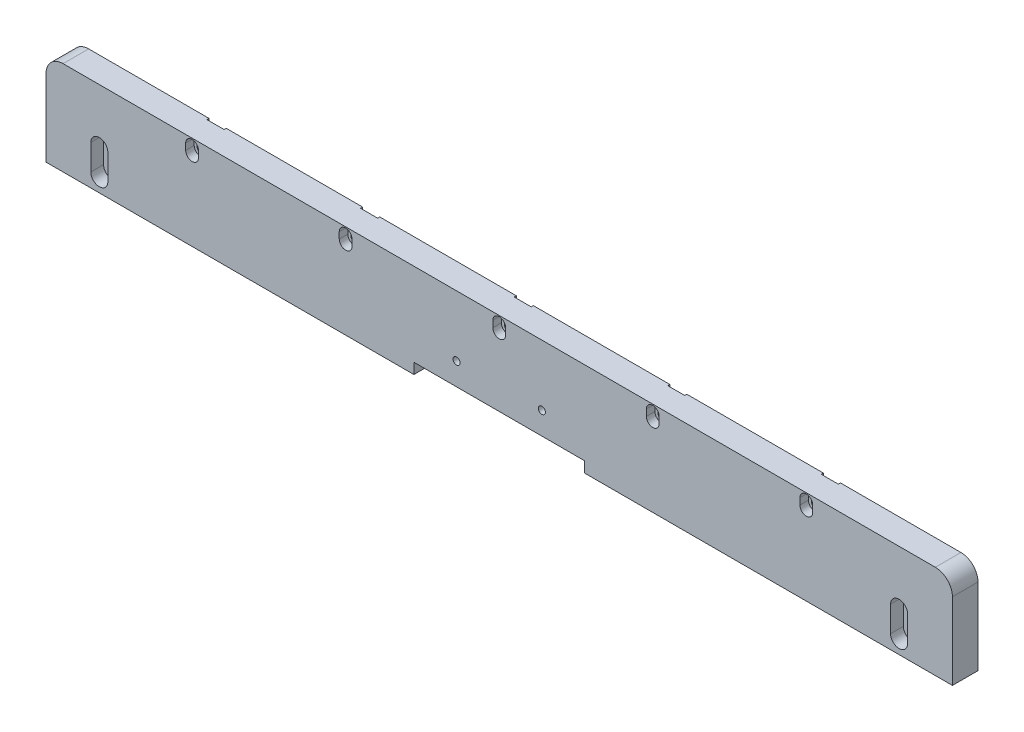
SolidWorks part; units mm, degrees
ref_plane "前视基准面" through (0, 0, 0) normal (0, 0, 1) x (1, 0, 0)
ref_plane "上视基准面" through (0, 0, 0) normal (0, 1, 0) x (1, 0, 0)
ref_plane "右视基准面" through (0, 0, 0) normal (1, 0, 0) x (0, 0, -1)
sketch "草图1" plane through (0, 0, 0) normal (0, 0, 1) x (1, 0, 0)
  line L1 (-212.5, 22) -> (212.5, 22)
  line L2 (-212.5, 22) -> (-212.5, -22)
  line L3 (-212.5, -22) -> (212.5, -22)
  line L4 (212.5, 22) -> (212.5, -22)
  line L5 (-212.5, 22) -> (212.5, -22) construction
  line L6 (-212.5, -22) -> (212.5, 22) construction
  point P0 (0, 0)
  dimension "D1" = 425
  dimension "D2" = 44
extrude "凸台-拉伸1" add sketch "草图1" along normal blind 12
fillet "圆角1" radius 8 2 edges at (212.5, 22, 6) (-212.5, 22, 6)
sketch "草图2" plane through (0, 0, 12) normal (0, 0, 1) x (1, 0, 0)
  line L0 (-187.5, -3.5) -> (-187.5, -15.5) construction
  line L1 (-183.5, -3.5) -> (-183.5, -15.5)
  line L2 (-191.5, -3.5) -> (-191.5, -15.5)
  line L3 (-212.5, 14) -> (-212.5, -22) construction
  line L4 (-212.5, -22) -> (212.5, -22) construction
  line L6 (0, 45.6197) -> (0, -20.1141) construction
  line L7 (187.5, -3.5) -> (187.5, -15.5) construction
  line L8 (183.5, -3.5) -> (183.5, -15.5)
  line L9 (191.5, -3.5) -> (191.5, -15.5)
  arc A0 (-183.5, -3.5) -> (-191.5, -3.5) centre (-187.5, -3.5) ccw
  arc A1 (-191.5, -15.5) -> (-183.5, -15.5) centre (-187.5, -15.5) ccw
  arc A2 (183.5, -3.5) -> (191.5, -3.5) centre (187.5, -3.5) cw
  arc A3 (191.5, -15.5) -> (183.5, -15.5) centre (187.5, -15.5) cw
  point P2 (-187.5, -9.5)
  point P16 (187.5, -9.5)
  dimension "D4" = 4
  dimension "D1" = 25
  dimension "D2" = 6.5
  dimension "D3" = 12
extrude "切除-拉伸1" cut sketch "草图2" against normal blind 6
sketch "草图3" plane through (0, 0, 6) normal (0, 0, 1) x (1, 0, 0)
  line L0 (-187.5, -3.5) -> (-187.5, -15.5) construction
  line L1 (-185.5, -3.5) -> (-185.5, -15.5)
  line L2 (-189.5, -3.5) -> (-189.5, -15.5)
  line L3 (187.5, -3.5) -> (187.5, -15.5) construction
  line L4 (189.5, -3.5) -> (189.5, -15.5)
  line L5 (185.5, -3.5) -> (185.5, -15.5)
  arc A0 (-185.5, -3.5) -> (-189.5, -3.5) centre (-187.5, -3.5) ccw
  arc A1 (-189.5, -15.5) -> (-185.5, -15.5) centre (-187.5, -15.5) ccw
  arc A2 (189.5, -3.5) -> (185.5, -3.5) centre (187.5, -3.5) ccw
  arc A3 (185.5, -15.5) -> (189.5, -15.5) centre (187.5, -15.5) ccw
  point P4 (-187.5, -9.5)
  point P13 (187.5, -9.5)
  dimension "D1" = 2
  dimension "D2" = 2
extrude "切除-拉伸2" cut sketch "草图3" against normal through all
sketch "草图8" plane through (0, 0, 12) normal (0, 0, 1) x (1, 0, 0)
  line L0 (-212.5, -22) -> (212.5, -22) construction
  line L1 (40, -17) -> (-40, -17)
  line L2 (40, -17) -> (40, -52.5185)
  line L3 (40, -52.5185) -> (-40, -52.5185)
  line L4 (-40, -17) -> (-40, -52.5185)
  line L5 (40, -17) -> (-40, -52.5185) construction
  line L6 (40, -52.5185) -> (-40, -17) construction
  line L7 (0, 36.33) -> (0, -6.1683) construction
  point P0 (0, -34.7592)
  point P10 (0, -17)
  dimension "D1" = 5
  dimension "D2" = 80
extrude "切除-拉伸3" cut sketch "草图8" against normal through all
sketch "草图10" plane through (0, 0, 0) normal (0, 0, -1) x (-1, 0, 0)
  line L0 (-204.5, 22) -> (204.5, 22) construction
  line L1 (-148, 22) -> (-140, 22)
  line L2 (-148, 22) -> (-148, 13.5)
  line L3 (-148, 13.5) -> (-140, 13.5)
  line L4 (-140, 22) -> (-140, 13.5)
  line L5 (-212.5, -22) -> (-212.5, 14) construction
  line L6 (-76, 22) -> (-76, 13.5)
  line L7 (-76, 22) -> (-68, 22)
  line L8 (-68, 22) -> (-68, 13.5)
  line L9 (-76, 13.5) -> (-68, 13.5)
  line L10 (-4, 22) -> (-4, 13.5)
  line L11 (-4, 22) -> (4, 22)
  line L12 (4, 22) -> (4, 13.5)
  line L13 (-4, 13.5) -> (4, 13.5)
  line L14 (68, 22) -> (68, 13.5)
  line L15 (68, 22) -> (76, 22)
  line L16 (76, 22) -> (76, 13.5)
  line L17 (68, 13.5) -> (76, 13.5)
  line L18 (140, 22) -> (140, 13.5)
  line L19 (140, 22) -> (148, 22)
  line L20 (148, 22) -> (148, 13.5)
  line L21 (140, 13.5) -> (148, 13.5)
  dimension "D1" = 64.5
  dimension "D2" = 8
  dimension "D3" = 8.5
extrude "切除-拉伸4" cut sketch "草图10" against normal blind 1
sketch "草图11" plane through (0, 0, 12) normal (0, 0, 1) x (1, 0, 0)
  line L0 (-144, 18.5) -> (-144, 15.5) construction
  line L1 (-141, 18.5) -> (-141, 15.5)
  line L2 (-147, 18.5) -> (-147, 15.5)
  line L3 (-212.5, 14) -> (-212.5, -22) construction
  line L4 (204.5, 22) -> (-204.5, 22) construction
  arc A0 (-141, 18.5) -> (-147, 18.5) centre (-144, 18.5) ccw
  arc A1 (-147, 15.5) -> (-141, 15.5) centre (-144, 15.5) ccw
  point P2 (-144, 17)
  dimension "D2" = 3
  dimension "D1" = 68.5
  dimension "D3" = 3
  dimension "D4" = 3.5
extrude "切除-拉伸5" cut sketch "草图11" against normal blind 4
sketch "草图12" plane through (0, 0, 8) normal (0, 0, 1) x (1, 0, 0)
  line L0 (-144, 18.5) -> (-144, 15.5) construction
  line L1 (-142.4, 18.5) -> (-142.4, 15.5)
  line L2 (-145.6, 18.5) -> (-145.6, 15.5)
  arc A0 (-142.4, 18.5) -> (-145.6, 18.5) centre (-144, 18.5) ccw
  arc A1 (-145.6, 15.5) -> (-142.4, 15.5) centre (-144, 15.5) ccw
  point P4 (-144, 17)
  dimension "D1" = 1.6
extrude "切除-拉伸6" cut sketch "草图12" against normal through all
pattern_linear "阵列(线性)1" count 5 spacing 72 along (1, 0, 0) of "切除-拉伸5", "切除-拉伸6"
hole_wizard "M4 螺纹孔1" positions "草图14" profile "草图13" tap size "M4" standard "Iso" end condition through all
sketch "草图14" plane through (0, 0, 12) normal (0, 0, 1) x (1, 0, 0)
  line L2 (-20, -6.5) -> (20, -6.5) construction
  line L4 (40, -17) -> (-40, -17) construction
  line L5 (0, 7.4507) -> (0, -3.3251) construction
  point P0 (-20, -6.5)
  point P2 (20, -6.5)
  point P23 (0, -6.5)
  dimension "D1" = 10.5
  dimension "D2" = 40
sketch "草图13" plane through (-20, -6.5, 12) normal (1, 0, 0) x (0, -1, 0)
  line L0 (0, 0) -> (0, 12)
  line L1 (0, 12) -> (1.65, 12)
  line L2 (1.65, 12) -> (1.65, 0)
  line L5 (1.65, 0) -> (0, 0)
  line L11 (0, -6.35) -> (0, 107.95) construction
  dimension "通孔螺纹孔钻头直径" = 3.3
  dimension "通孔螺纹孔钻头深度" = 12
cosmetic thread "孔螺蚊线1" parameters "D2"=4
cosmetic thread "孔螺蚊线2" parameters "D2"=4
